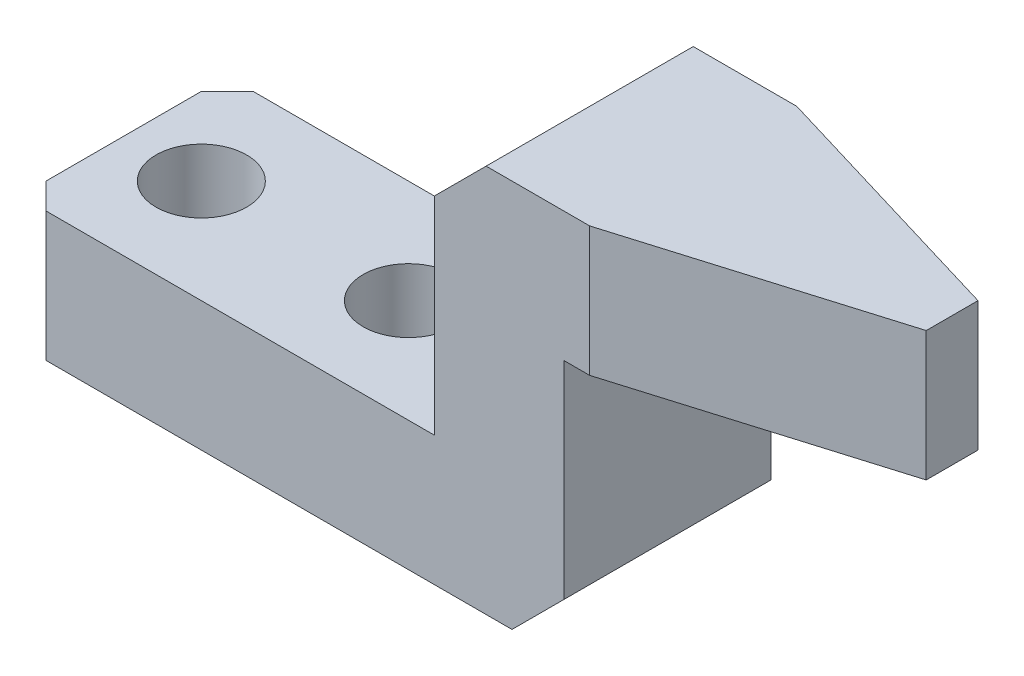
from build123d import *

# Parameters (mm, degrees)
SKETCH1_W                  = 32
SKETCH1_H                  = 15
BOSS_EXTRUDE1_DEPTH        = 4
SKETCH2_W                  = 16
SKETCH2_H                  = 10
SKETCH2_W_2                = 11
CUT_EXTRUDE1_DEPTH         = 20.397164741
CHAMFER1_SIZE              = 1
CHAMFER2_SIZE              = 2
F_3_5_3_5_DIAMETER_HOLE1_D = 3.5
CHAMFER3_SIZE              = 3
CHAMFER3_SIZE2             = 10
CHAMFER4_SIZE              = 10
CHAMFER4_SIZE2             = 3


with BuildPart() as part:
    # Sketch1 → Boss-Extrude1 (new, symmetric)
    with BuildSketch(Plane.XY):
        Rectangle(SKETCH1_W, SKETCH1_H)
    extrude(amount=BOSS_EXTRUDE1_DEPTH, both=True)

    # Sketch2 → Cut-Extrude1 (cut, through all)
    with BuildSketch(Plane.XY.offset(4)):
        with Locations((-8, 2.5)):
            Rectangle(SKETCH2_W, SKETCH2_H)
        with Locations((10.5, -2.5)):
            Rectangle(SKETCH2_W_2, SKETCH2_H)
    extrude(amount=-CUT_EXTRUDE1_DEPTH, mode=Mode.SUBTRACT)

    # Chamfer1
    chamfer1_edges = [part.edges().sort_by_distance(p)[0] for p in [
        (-16, -5, -4),
        (-16, -5, 4),
    ]]
    chamfer(chamfer1_edges, length=CHAMFER1_SIZE)

    # Chamfer2
    chamfer2_edges = [part.edges().sort_by_distance(p)[0] for p in [
        (0, 7.5, 0),
        (5, -7.5, 0),
    ]]
    chamfer(chamfer2_edges, length=CHAMFER2_SIZE)

    # Ø3.5 (3.5) Diameter Hole1 (through all)
    with Locations(Plane(origin=(0, -2.5, 0), x_dir=(1, 0, 0), z_dir=(0, 1, 0))):
        with Locations((-13, 0), (-5, 0)):
            Hole(F_3_5_3_5_DIAMETER_HOLE1_D / 2)

    # Chamfer3
    chamfer3_edges = [part.edges().sort_by_distance(p)[0] for p in [
        (16, 5, 4),
    ]]
    chamfer3_side = [part.faces().sort_by_distance(p)[0] for p in [
        (16, 5, 0),
    ]]
    chamfer(chamfer3_edges, length=CHAMFER3_SIZE, length2=CHAMFER3_SIZE2, reference=chamfer3_side[0])

    # Chamfer4
    chamfer4_edges = [part.edges().sort_by_distance(p)[0] for p in [
        (16, 5, -4),
    ]]
    chamfer4_side = [part.faces().sort_by_distance(p)[0] for p in [
        (0.957711443, -0.497512438, -4),
    ]]
    chamfer(chamfer4_edges, length=CHAMFER4_SIZE, length2=CHAMFER4_SIZE2, reference=chamfer4_side[0])


solid = part.part
